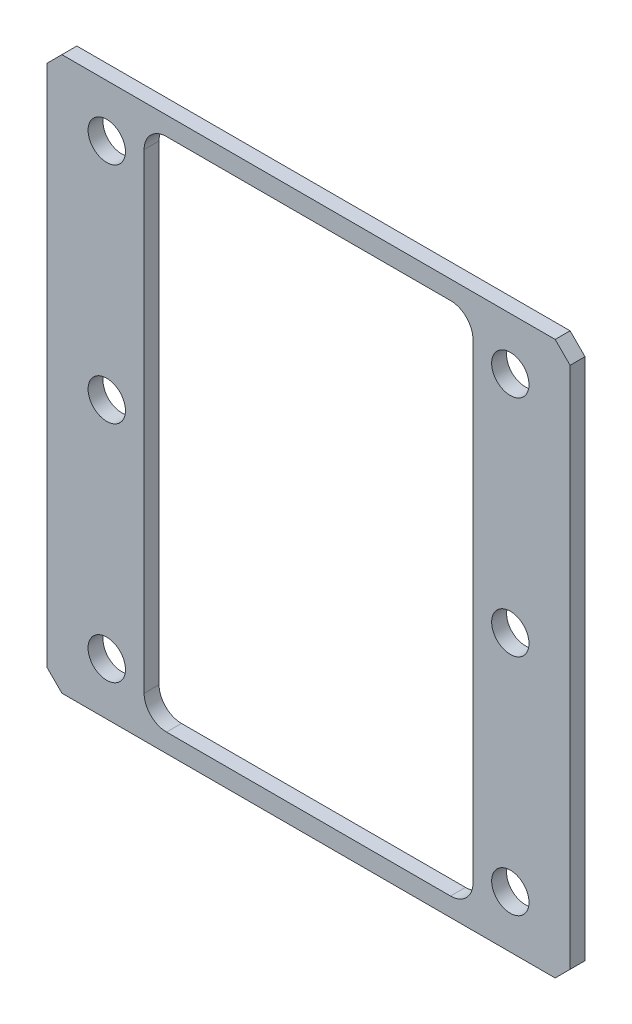
from build123d import *

# Parameters (mm, degrees)
SKETCH1_W           = 70
SKETCH1_H           = 74
SKETCH1_R           = 2.5
BOSS_EXTRUDE1_DEPTH = 2
CHAMFER1_SIZE       = 2


with BuildPart() as part:
    # Sketch1 → Boss-Extrude1 (new body)
    with BuildSketch(Plane.XY):
        Rectangle(SKETCH1_W, SKETCH1_H)
        with Locations((-27, 30)):
            Circle(SKETCH1_R, mode=Mode.SUBTRACT)
        with Locations((-27, 0)):
            Circle(SKETCH1_R, mode=Mode.SUBTRACT)
        with Locations((-27, -30)):
            Circle(SKETCH1_R, mode=Mode.SUBTRACT)
        with Locations((27, -30)):
            Circle(SKETCH1_R, mode=Mode.SUBTRACT)
        with Locations((27, 0)):
            Circle(SKETCH1_R, mode=Mode.SUBTRACT)
        with Locations((27, 30)):
            Circle(SKETCH1_R, mode=Mode.SUBTRACT)
        with BuildLine():
            Line((-19, -34.5), (19, -34.5))
            ThreePointArc((19, -34.5), (21.121320344, -33.621320344), (22, -31.5))
            Line((22, -31.5), (22, 31.5))
            ThreePointArc((22, 31.5), (21.121320344, 33.621320344), (19, 34.5))
            Line((19, 34.5), (-19, 34.5))
            ThreePointArc((-19, 34.5), (-21.121320344, 33.621320344), (-22, 31.5))
            Line((-22, 31.5), (-22, -31.5))
            ThreePointArc((-22, -31.5), (-21.121320344, -33.621320344), (-19, -34.5))
        make_face(mode=Mode.SUBTRACT)
    extrude(amount=BOSS_EXTRUDE1_DEPTH)

    # Chamfer1
    chamfer1_edges = [part.edges().sort_by_distance(p)[0] for p in [
        (35, -37, 1),
        (-35, -37, 1),
        (-35, 37, 1),
        (35, 37, 1),
    ]]
    chamfer(chamfer1_edges, length=CHAMFER1_SIZE)


solid = part.part
